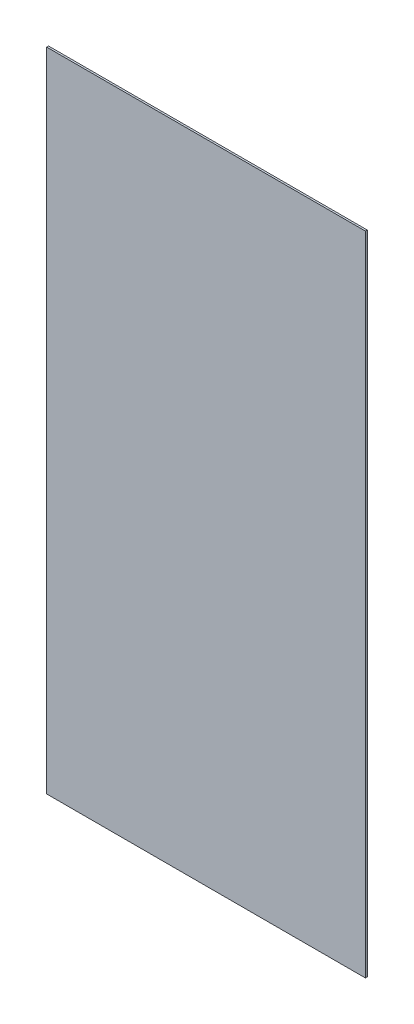
from build123d import *

# Parameters (mm, degrees)
SKETCH_1_W      = 340
SKETCH_1_H      = 690
EXTRUDE_1_DEPTH = 2


with BuildPart() as part:
    # 草图1 → 凸台-拉伸1 (new body)
    with BuildSketch(Plane.XY):
        with Locations((-81.402439024, -174.115853659)):
            Rectangle(SKETCH_1_W, SKETCH_1_H)
    extrude(amount=EXTRUDE_1_DEPTH)


solid = part.part
